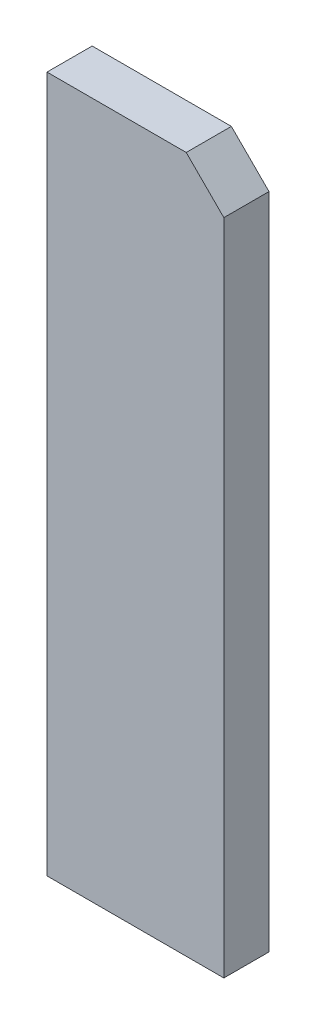
SolidWorks part; units mm, degrees
ref_plane "前视基准面" through (0, 0, 0) normal (0, 0, 1) x (1, 0, 0)
ref_plane "上视基准面" through (0, 0, 0) normal (0, 1, 0) x (1, 0, 0)
ref_plane "右视基准面" through (0, 0, 0) normal (1, 0, 0) x (0, 0, -1)
sketch "草图1" plane through (0, 0, 0) normal (0, 0, 1) x (1, 0, 0)
  line L0 (0, 0) -> (47, 0)
  line L1 (47, 0) -> (47, 185)
  line L2 (47, 185) -> (0, 185)
  line L3 (0, 185) -> (0, 0)
  dimension "D1" = 47
  dimension "D2" = 185
extrude "凸台-拉伸1" add sketch "草图1" along normal mid plane 12
sketch "草图2" plane through (0, 0, 6) normal (0, 0, 1) x (1, 0, 0)
  line L0 (0, 0) -> (47, 0) construction
  line L1 (35, 165) -> (12, 165)
  line L2 (35, 165) -> (35, 12)
  line L3 (35, 12) -> (12, 12)
  line L4 (12, 165) -> (12, 12)
  line L5 (0, 185) -> (0, 0) construction
  line L6 (47, 0) -> (47, 185) construction
  line L7 (47, 185) -> (0, 185) construction
  dimension "D1" = 12
  dimension "D2" = 12
  dimension "D3" = 12
  dimension "D4" = 20
chamfer "倒角1" distance 10 angle 45 1 edges at (47, 185, 0)
extrude "切除-拉伸1" [suppressed] cut sketch "草图2" against normal up to next
fillet "圆角1" [suppressed] radius 2
